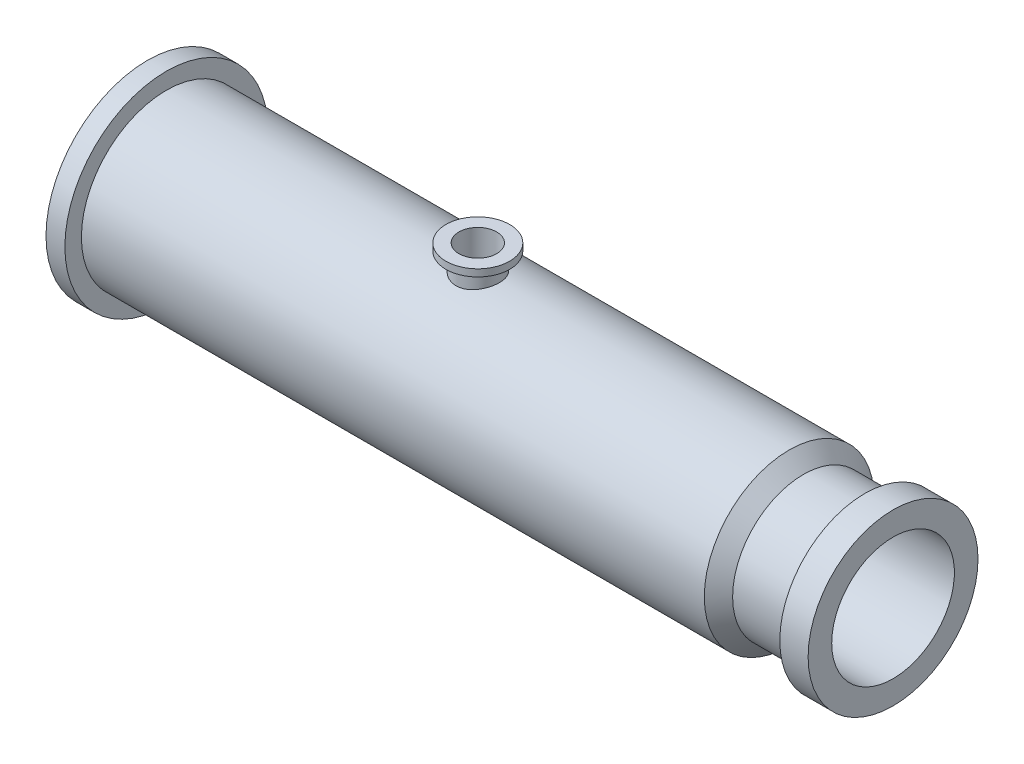
from build123d import *

# Parameters (mm, degrees)
SKETCH3_R           = 46
SKETCH3_R_2         = 40
BOSS_EXTRUDE1_DEPTH = 215
SKETCH4_R           = 160
CUT_EXTRUDE1_DEPTH  = 900
CUT_EXTRUDE2_START  = -300
SKETCH5_R           = 40
CUT_EXTRUDE2_DEPTH  = 300
SKETCH6_R           = 67.5
SKETCH6_R_2         = 40
BOSS_EXTRUDE2_DEPTH = 15


with BuildPart() as part:
    # Sketch1 → Revolve1 (revolve)
    with BuildSketch(Plane.XY, mode=Mode.PRIVATE) as revolve1_sk:
        Polygon((0, 160), (0, 215), (40, 215), (40, 180), (1360, 180), (1390, 150), (1520, 150), (1520, 180), (1580, 180), (1580, 130), (1381.715728753, 130), (1351.715728753, 160), align=None)
    revolve(revolve1_sk.sketch.rotate(Axis((0, 0, 0), (1, 0, 0)), 90), axis=Axis((0, 0, 0), (1, 0, 0)))

    # Sketch3 → Boss-Extrude1 (add)
    with BuildSketch(Plane(origin=(0, 0, 0), x_dir=(1, 0, 0), z_dir=(0, 1, 0))):
        with Locations(Location((700, 0, 0), (0, 0, 90))):
            Circle(SKETCH3_R)
        with Locations(Location((700, 0, 0), (0, 0, 90))):
            Circle(SKETCH3_R_2, mode=Mode.SUBTRACT)
    extrude(amount=BOSS_EXTRUDE1_DEPTH)

    # Sketch4 → Cut-Extrude1 (cut)
    with BuildSketch(Plane.ZY):
        Circle(SKETCH4_R)
    extrude(amount=-CUT_EXTRUDE1_DEPTH, mode=Mode.SUBTRACT)

    # Sketch5 → Cut-Extrude2 (cut)
    with BuildSketch(Plane(origin=(0, 215, 0), x_dir=(1, 0, 0), z_dir=(0, 1, 0)).offset(CUT_EXTRUDE2_START)):
        with Locations(Location((700, 0, 0), (0, 0, 270))):
            Circle(SKETCH5_R)
    extrude(amount=CUT_EXTRUDE2_DEPTH, mode=Mode.SUBTRACT)

    # Sketch6 → Boss-Extrude2 (add)
    with BuildSketch(Plane(origin=(0, 215, 0), x_dir=(1, 0, 0), z_dir=(0, 1, 0))):
        with Locations(Location((700, 0, 0), (0, 0, 270))):
            Circle(SKETCH6_R)
        with Locations(Location((700, 0, 0), (0, 0, 270))):
            Circle(SKETCH6_R_2, mode=Mode.SUBTRACT)
    extrude(amount=BOSS_EXTRUDE2_DEPTH)


solid = part.part
